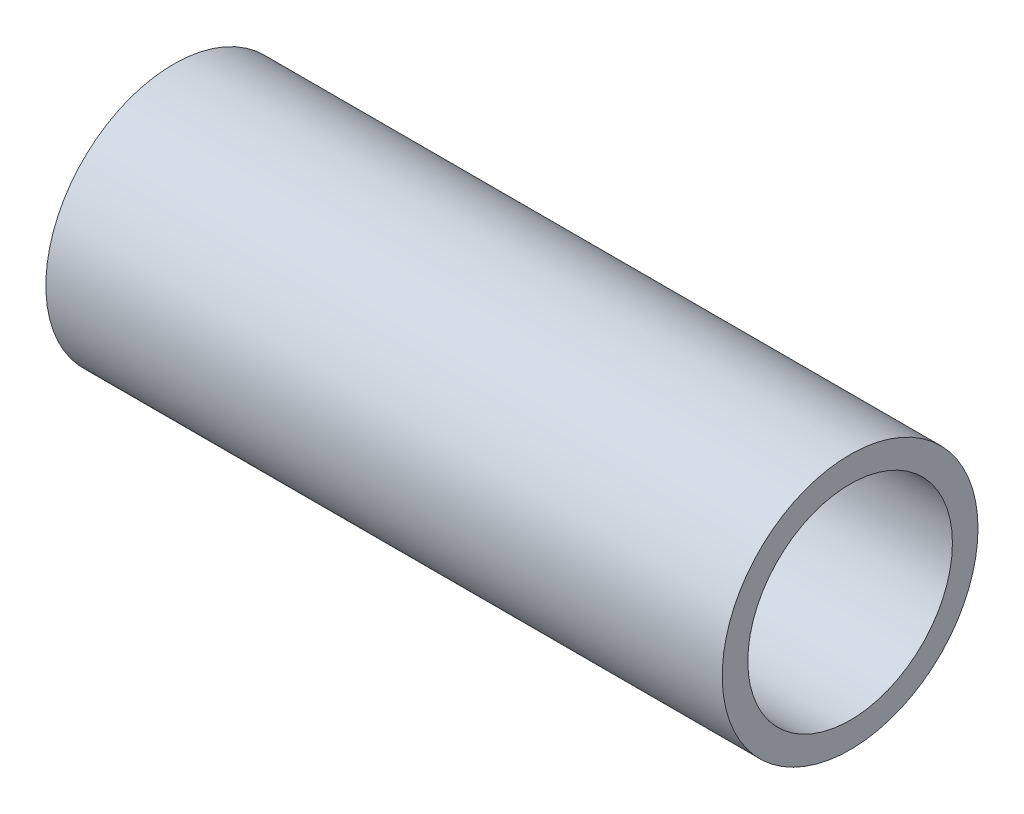
from build123d import *

# Parameters (mm, degrees)
SKETCH_1_R      = 22.5
SKETCH_1_R_2    = 18
EXTRUDE_1_DEPTH = 119


with BuildPart() as part:
    # 草图1 → 凸台-拉伸1 (new body)
    with BuildSketch(Plane(origin=(0, 0, 0), x_dir=(0, 0, -1), z_dir=(1, 0, 0))):
        Circle(SKETCH_1_R)
        Circle(SKETCH_1_R_2, mode=Mode.SUBTRACT)
    extrude(amount=EXTRUDE_1_DEPTH)


solid = part.part
